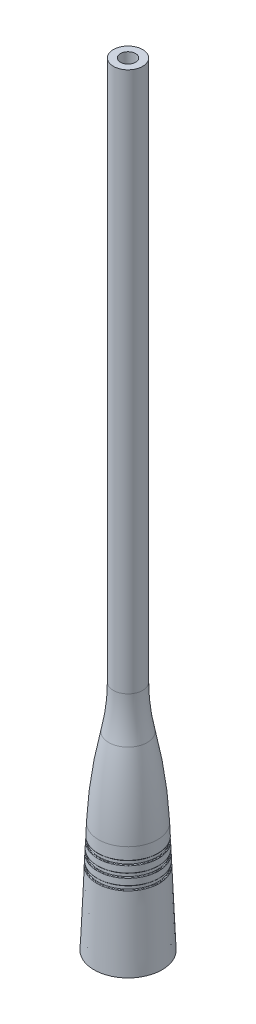
SolidWorks part; units mm, degrees
material "ABS"
ref_plane "前视基准面" through (0, 0, 0) normal (0, 0, 1) x (1, 0, 0)
ref_plane "上视基准面" through (0, 0, 0) normal (0, 1, 0) x (1, 0, 0)
ref_plane "右视基准面" through (0, 0, 0) normal (1, 0, 0) x (0, 0, -1)
sketch "草图1" plane through (0, 0, 0) normal (0, 0, 1) x (1, 0, 0)
  line L0 (0, 0) -> (0, 176.7014) construction
  line L1 (-7.4, 0) -> (-6.7333, 16)
  line L2 (-3.175, 50.5) -> (-3.175, 168)
  line L3 (-7.4, 0) -> (-6.2, 0)
  line L4 (-6.2, 0) -> (-6.2, 2.5)
  line L5 (-6.2, 2.5) -> (-4.75, 2.5)
  line L6 (-4.75, 2.5) -> (-4.75, 10.5)
  line L7 (-4.75, 10.5) -> (-3.75, 10.5)
  line L8 (-3.75, 10.5) -> (-3.75, 40)
  line L9 (-3.75, 40) -> (-1.65, 40)
  line L10 (-1.65, 40) -> (-1.65, 168)
  line L11 (-1.65, 168) -> (-3.175, 168)
  line L12 (-6.5083, 21.4) -> (-6.2581, 21.4)
  line L13 (-6.2914, 20.6) -> (-6.2581, 21.4)
  line L14 (-6.2914, 20.6) -> (-6.5417, 20.6)
  line L15 (-6.6042, 19.1) -> (-6.3539, 19.1)
  line L16 (-6.3873, 18.3) -> (-6.3539, 19.1)
  line L17 (-6.3873, 18.3) -> (-6.6375, 18.3)
  line L18 (-6.7, 16.8) -> (-6.4498, 16.8)
  line L19 (-6.4831, 16) -> (-6.4498, 16.8)
  line L20 (-6.4831, 16) -> (-6.7333, 16)
  line L21 (-6.5083, 21.4) -> (-6.4, 24)
  line L22 (-6.6042, 19.1) -> (-6.5417, 20.6)
  line L23 (-6.7, 16.8) -> (-6.6375, 18.3)
  arc A0 (-6.4, 24) -> (-4.1807, 41.1884) centre (93.5133, 19.8369) cw
  arc A1 (-4.1807, 41.1884) -> (-3.175, 50.5) centre (-46.7859, 50.5) ccw
  dimension "D1" = 14.8
  dimension "D4" = 50.5
  dimension "D6" = 12.8
  dimension "D7" = 100
  dimension "D2" = 24
  dimension "D3" = 168
  dimension "D5" = 6.35
  dimension "D8" = 12.4
  dimension "D9" = 2.5
  dimension "D10" = 9.5
  dimension "D11" = 10.5
  dimension "D12" = 7.5
  dimension "D13" = 3.3
  dimension "D14" = 0.25
  dimension "D15" = 1.5
  dimension "D16" = 1.5
  dimension "D17" = 16
  dimension "D18" = 40
revolve "旋转1" add sketch "草图1" angle 360 about L0
fillet "圆角3" radius 0.1 12 edges at (0, 21.4, -6.2581) (0, 21.4, -6.5083) (0, 20.6, -6.2914) (0, 20.6, -6.5417) (0, 19.1, -6.3539) (0, 19.1, -6.6042) (0, 18.3, -6.3873) (0, 18.3, -6.6375) (0, 16.8, -6.4498) (0, 16.8, -6.7) (0, 16, -6.4831) (0, 16, -6.7333)
